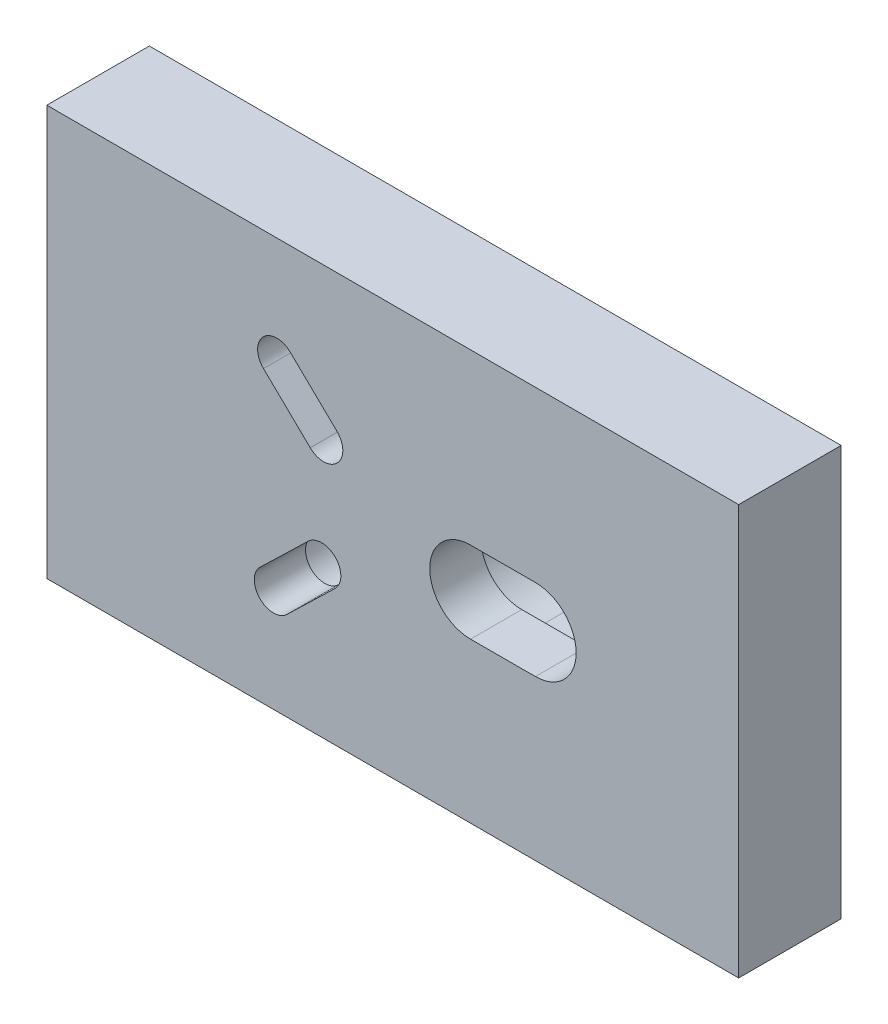
SolidWorks part; units mm, degrees
ref_plane "前视基准面" through (0, 0, 0) normal (0, 0, 1) x (1, 0, 0)
ref_plane "上视基准面" through (0, 0, 0) normal (0, 1, 0) x (1, 0, 0)
ref_plane "右视基准面" through (0, 0, 0) normal (1, 0, 0) x (0, 0, -1)
sketch "草图1" plane through (0, 0, 0) normal (0, 0, 1) x (1, 0, 0)
  line L1 (-9.6011, 4.1182) -> (17.3989, 4.1182)
  line L2 (-9.6011, 4.1182) -> (-9.6011, -11.8818)
  line L3 (-9.6011, -11.8818) -> (17.3989, -11.8818)
  line L4 (17.3989, 4.1182) -> (17.3989, -11.8818)
  dimension "D1" = 27
  dimension "D2" = 16
extrude "凸台-拉伸1" add sketch "草图1" along normal blind 4
sketch "草图2" plane through (0, 0, 4) normal (0, 0, 1) x (1, 0, 0)
  circle A0 centre (1.1999, -1.7816) radius 0.75
  circle A1 centre (1.1225, -6.0568) radius 0.75
  circle A2 centre (9.4654, -4.0695) radius 1.59
extrude "切除-拉伸2" cut sketch "草图2" against normal up to surface (4 mm away) up to face at (3.8989, -3.8818, 0)
sketch "草图3" plane through (0, 0, 4) normal (0, 0, 1) x (1, 0, 0)
  line L0 (6.9319, -2.4815) -> (9.4642, -2.4795)
  line L1 (6.9343, -5.6615) -> (9.4666, -5.6595)
  line L2 (-1.2764, -7.3328) -> (0.6012, -5.5176)
  line L3 (1.6438, -6.596) -> (-0.2339, -8.4112)
  line L4 (-1.146, -0.5569) -> (0.6786, -2.3208)
  line L5 (1.7212, -1.2424) -> (-0.1034, 0.5215)
  arc A0 (6.9319, -2.4815) -> (6.9343, -5.6615) centre (6.9331, -4.0715) ccw
  arc A1 (1.7212, -1.2424) -> (0.6786, -2.3208) centre (1.1999, -1.7816) ccw
  arc A2 (0.6012, -5.5176) -> (1.6438, -6.596) centre (1.1225, -6.0568) ccw
  arc A3 (-0.1034, 0.5215) -> (-1.146, -0.5569) centre (-0.6247, -0.0177) ccw
  arc A4 (-1.2764, -7.3328) -> (-0.2339, -8.4112) centre (-0.7552, -7.872) ccw
  arc A5 (9.4642, -2.4795) -> (9.4666, -5.6595) centre (9.4654, -4.0695) ccw
extrude "切除-拉伸3" cut sketch "草图3" against normal up to surface (4 mm away) up to face at (11.0554, -4.0695, 0)
ref_plane "基准面1" through (6.0939, -7.0568, 27.9723) normal (0.0574, 0.9942, -0.0909) x (0.9983, -0.0572, 0.0052)
sketch "草图5" plane through (0, 0, 0) normal (0, 0, -1) x (-1, 0, 0)
  line L0 (-9.4635, -1.5695) -> (-6.9312, -1.5715)
  line L1 (-9.4673, -6.5695) -> (-6.935, -6.5715)
  line L2 (-0.2441, 0.881) -> (-2.0687, -0.8829)
  line L3 (-0.3311, -2.6803) -> (1.4935, -0.9164)
  line L4 (-0.2537, -5.1581) -> (1.624, -6.9733)
  line L5 (-1.9913, -6.9555) -> (-0.1136, -8.7707)
  arc A0 (-9.4635, -1.5695) -> (-9.4673, -6.5695) centre (-9.4654, -4.0695) ccw
  arc A1 (-6.935, -6.5715) -> (-6.9312, -1.5715) centre (-6.9331, -4.0715) ccw
  arc A2 (-2.0687, -0.8829) -> (-0.3311, -2.6803) centre (-1.1999, -1.7816) ccw
  arc A3 (1.4935, -0.9164) -> (-0.2441, 0.881) centre (0.6247, -0.0177) ccw
  arc A4 (-0.2537, -5.1581) -> (-1.9913, -6.9555) centre (-1.1225, -6.0568) ccw
  arc A5 (-0.1136, -8.7707) -> (1.624, -6.9733) centre (0.7552, -7.872) ccw
extrude "切除-拉伸4" cut sketch "草图5" against normal blind 2
